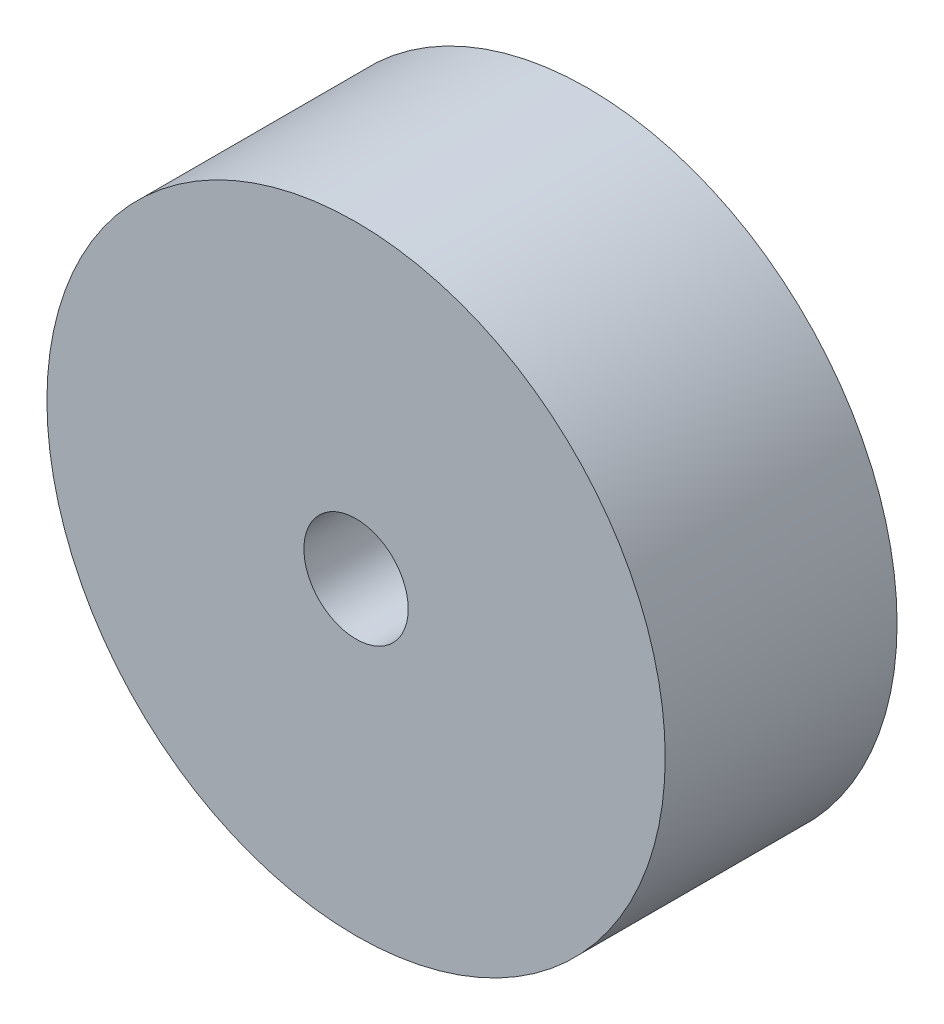
SolidWorks part; units mm, degrees
material "普通碳钢"
ref_plane "Front Plane" through (0, 0, 0) normal (0, 0, 1) x (1, 0, 0)
ref_plane "Top Plane" through (0, 0, 0) normal (0, 1, 0) x (1, 0, 0)
ref_plane "Right Plane" through (0, 0, 0) normal (1, 0, 0) x (0, 0, -1)
sketch "草图1" plane through (0, 0, 0) normal (0, 0, 1) x (1, 0, 0)
  circle A0 centre (0, 0) radius 24
  circle A1 centre (0, 0) radius 4.05
  dimension "D1" = 8.1
  dimension "D2" = 48
extrude "凸台-拉伸1" add sketch "草图1" along normal blind 18
